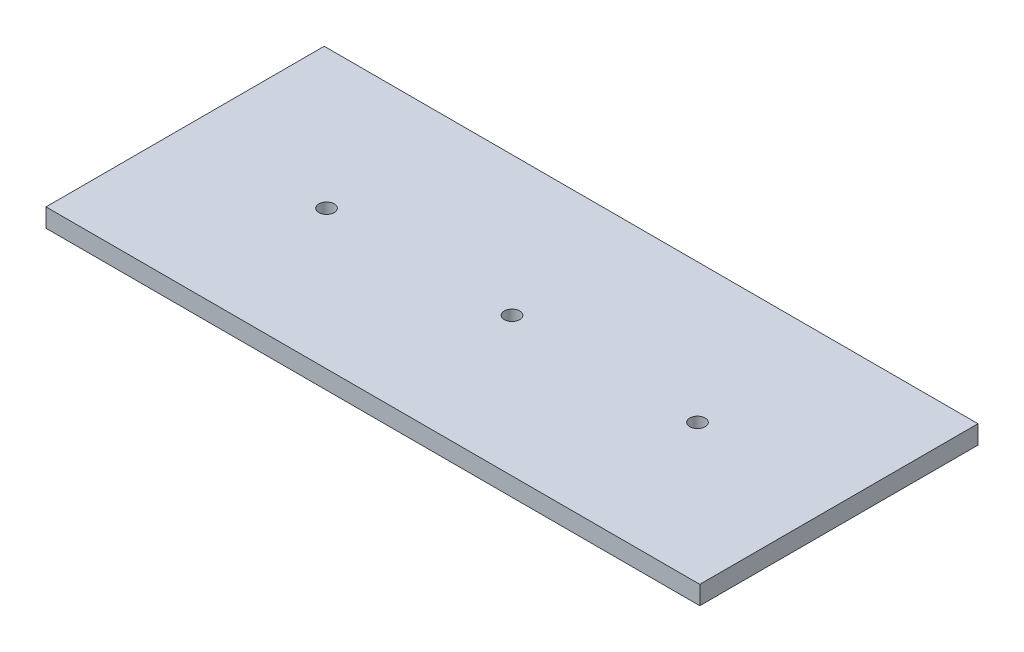
from build123d import *

# Parameters (mm, degrees)
SKETCH1_W           = 141
SKETCH1_H           = 60
BOSS_EXTRUDE1_DEPTH = 4
M4_TAPPED_HOLE1_D   = 3.3


with BuildPart() as part:
    # Sketch1 → Boss-Extrude1 (new body)
    with BuildSketch(Plane(origin=(0, 0, 0), x_dir=(1, 0, 0), z_dir=(0, 1, 0))):
        Rectangle(SKETCH1_W, SKETCH1_H)
    extrude(amount=BOSS_EXTRUDE1_DEPTH)

    # M4 Tapped Hole1 (through all)
    with Locations(Plane(origin=(0, 4, 0), x_dir=(1, 0, 0), z_dir=(0, 1, 0))):
        with Locations((-40, 0), (0, 0), (40, 0)):
            Hole(M4_TAPPED_HOLE1_D / 2)


solid = part.part
